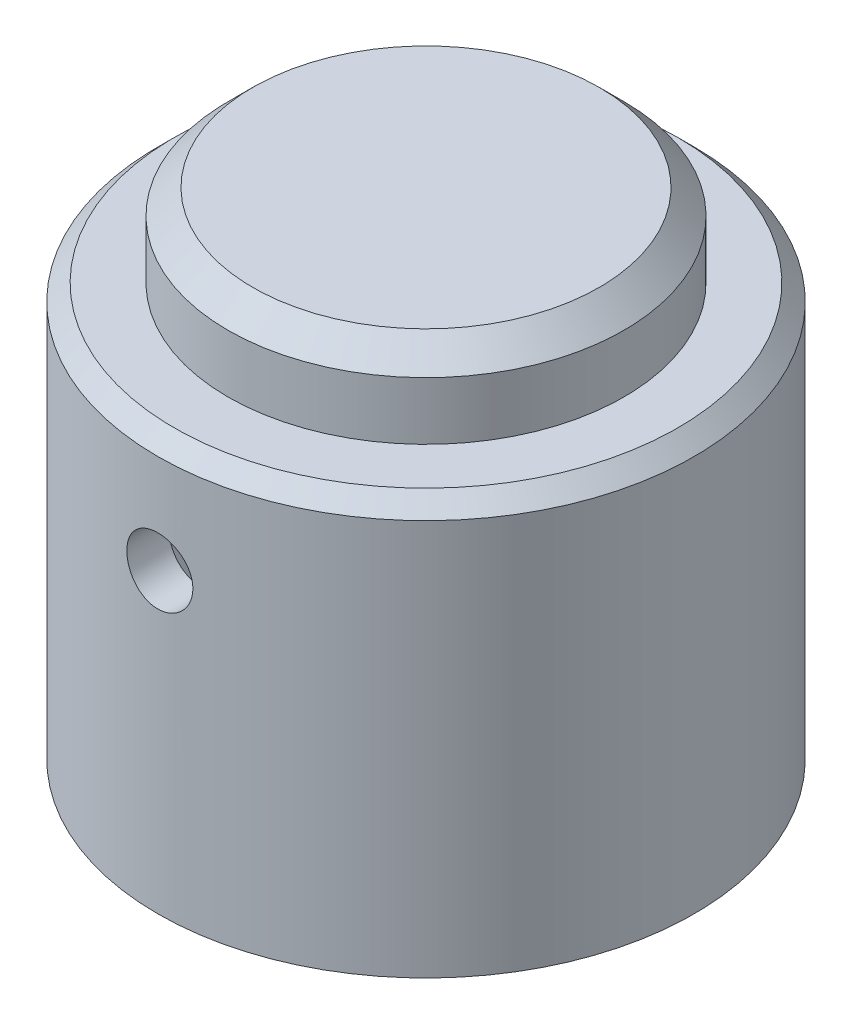
from build123d import *

# Parameters (mm, degrees)
CHAMFER1_SIZE      = 3
CHAMFER2_SIZE      = 2
CUT_EXTRUDE1_START = -20
SKETCH3_R          = 4
CUT_EXTRUDE1_DEPTH = 105
CUT_EXTRUDE2_START = 125
SKETCH4_R          = 4
CUT_EXTRUDE2_DEPTH = 105


with BuildPart() as part:
    # Sketch1 → Revolve1 (revolve)
    with BuildSketch(Plane.XY, mode=Mode.PRIVATE) as revolve1_sk:
        Polygon((0, 60), (-24, 60), (-24, 50), (-32.5, 50), (-32.5, 0), (0, 0), align=None)
    revolve(revolve1_sk.sketch.rotate(Axis((0, 0, 0), (0, 1, 0)), 270), axis=Axis((0, 0, 0), (0, 1, 0)))

    # Chamfer1
    chamfer1_edges = [part.edges().sort_by_distance(p)[0] for p in [
        (0, 60, 24),
    ]]
    chamfer(chamfer1_edges, length=CHAMFER1_SIZE)

    # Chamfer2
    chamfer2_edges = [part.edges().sort_by_distance(p)[0] for p in [
        (0, 50, 32.5),
    ]]
    chamfer(chamfer2_edges, length=CHAMFER2_SIZE)

    # Sketch2 → Cut-Revolve1 (revolve, cut)
    with BuildSketch(Plane.XY):
        Polygon((-27.5, 0), (-27.5, 40), (-15, 40), (-15, 38), (0, 38), (0, 0), align=None)
    revolve(axis=Axis((0, 38, 0), (0, -1, 0)), mode=Mode.SUBTRACT)

    # Sketch3 → Cut-Extrude1 (cut)
    with BuildSketch(Plane.XY.offset(CUT_EXTRUDE1_START)):
        with Locations(Location((0, 36, 0), (0, 0, 90))):
            Circle(SKETCH3_R)
    extrude(amount=-CUT_EXTRUDE1_DEPTH, mode=Mode.SUBTRACT)

    # Sketch4 → Cut-Extrude2 (cut)
    with BuildSketch(Plane.XY.offset(CUT_EXTRUDE2_START)):
        with Locations(Location((0, 36, 0), (0, 0, 90))):
            Circle(SKETCH4_R)
    extrude(amount=-CUT_EXTRUDE2_DEPTH, mode=Mode.SUBTRACT)

    # Sketch7 → Cut-Revolve2 (revolve, cut)
    with BuildSketch(Plane(origin=(0, 0, 0), x_dir=(0, 0, -1), z_dir=(1, 0, 0)), mode=Mode.PRIVATE) as cut_revolve2_sk:
        Polygon((-5.375, 38), (-5.375, 50), (0, 53.103257697), (0, 38), align=None)
    revolve(cut_revolve2_sk.sketch.rotate(Axis((0, 53.103257697, 0), (0, -1, 0)), 180), axis=Axis((0, 53.103257697, 0), (0, -1, 0)), mode=Mode.SUBTRACT)


solid = part.part
